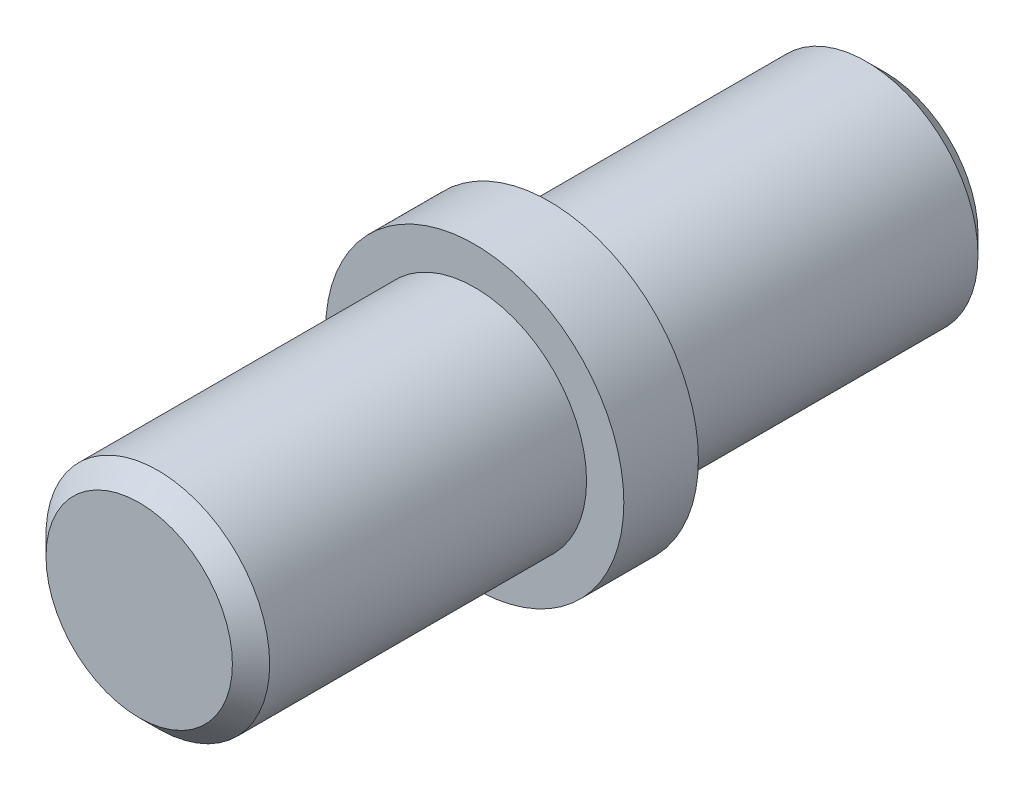
SolidWorks part; units mm, degrees
material "碳钢镀锌"
ref_plane "前视" through (0, 0, 0) normal (0, 0, 1) x (1, 0, 0)
ref_plane "上视" through (0, 0, 0) normal (0, 1, 0) x (1, 0, 0)
ref_plane "右视" through (0, 0, 0) normal (1, 0, 0) x (0, 0, -1)
sketch "草图1" plane through (0, 0, 0) normal (0, 0, 1) x (1, 0, 0)
  circle A0 centre (0, 0) radius 4
  dimension "D1" = 8
extrude "凸台-拉伸1" add sketch "草图1" along normal mid plane 2 contours A0
sketch "草图2" plane through (0, 0, 1) normal (0, 0, 1) x (1, 0, 0)
  circle A0 centre (0, 0) radius 3
  dimension "D1" = 6
extrude "凸台-拉伸2" add sketch "草图2" along normal blind 9 contours A0
mirror "镜向5" about plane through (0, 0, 0) normal (0, 0, 1) of "凸台-拉伸2"
chamfer "倒角1" distance 0.5 angle 45 2 edges at (3, 0, 10) (3, 0, -10)
